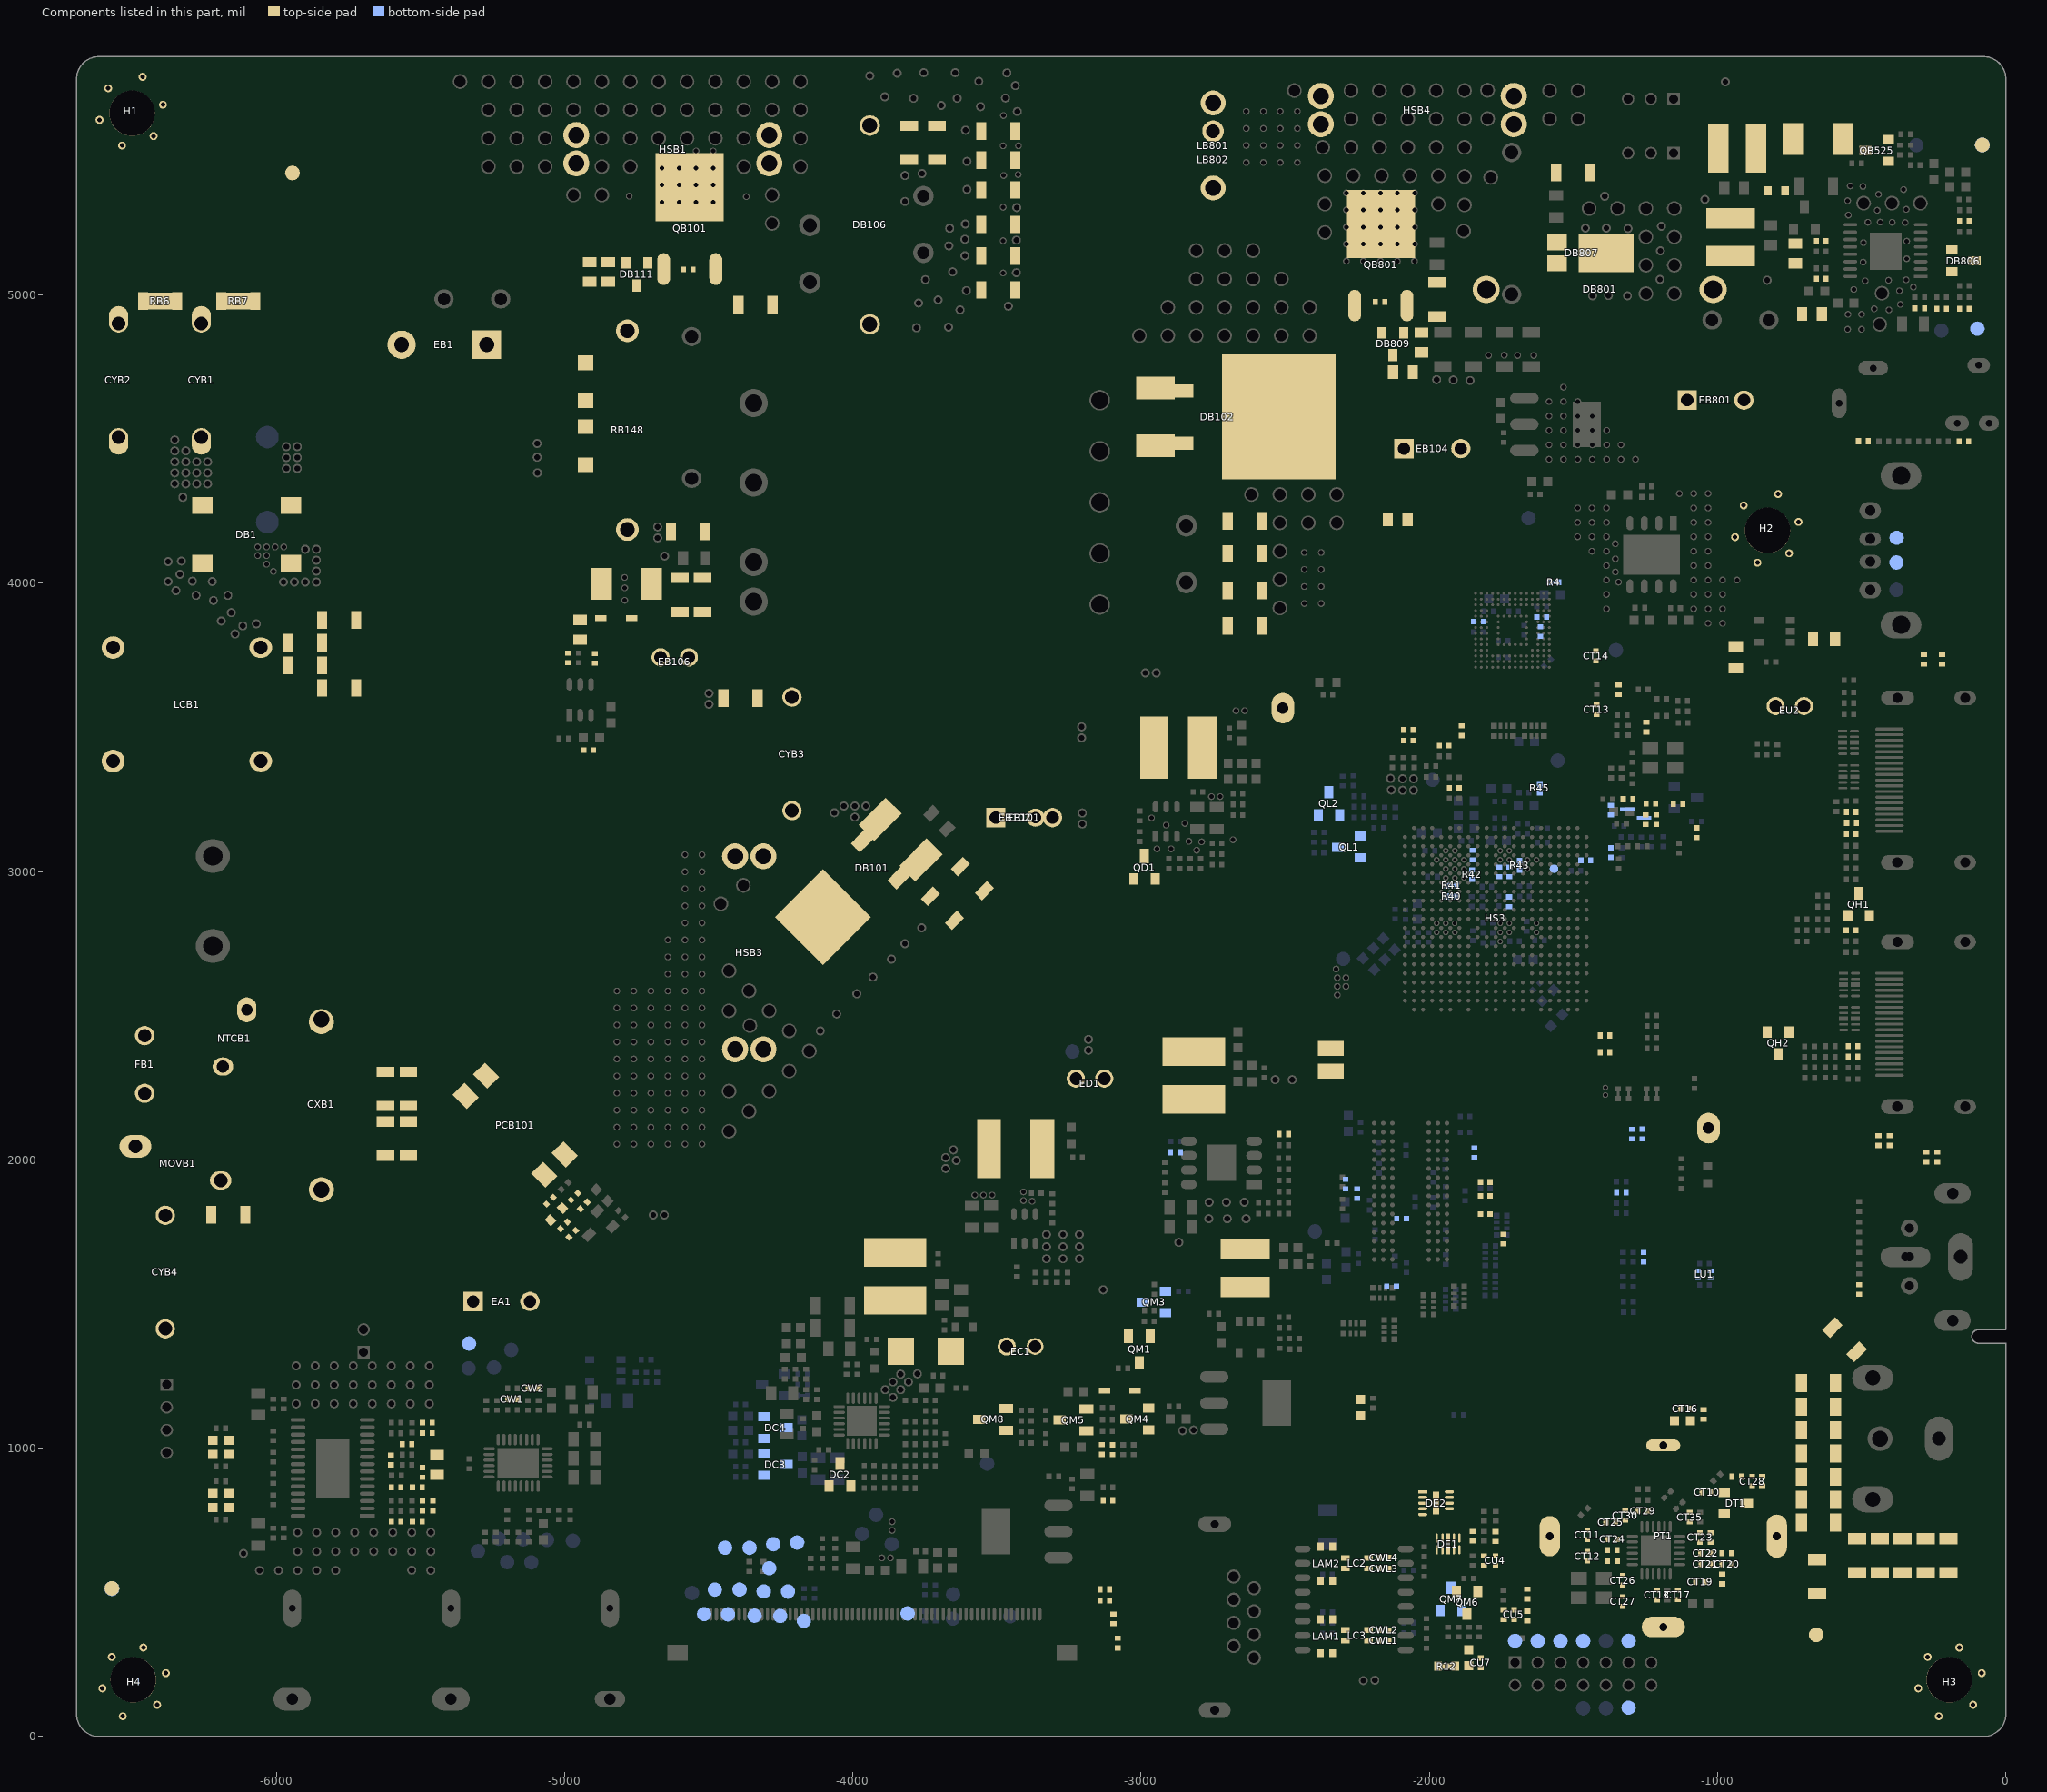
[diagram p0: the components of this part, seen from the top]
# Altium PCB MISC84395.PcbDoc (part 3 of 26)
Units mil, origin at the board's own origin, x right, y up, seen from the top; angles counter-clockwise.
Board outline 6692.91 x 5826.77 mil, 2 copper layers (TopLayer, BottomLayer), stack 61.855 mil thick; 951 components, 565 nets, 4374 pads, 1804 vias.
Unrouted connection lines stored in the file: 1.

## Components (designator, comment, footprint, x,y, rotation, side; value= is the part's Value field where it differs from the comment) (continued)
CT10 "0.1uF-0402-X5R-±20%-16V" C0402#1 -1037.15,847 r180 top
CT11 "30pF-0402-NPO-±5%-50V" C0402#1 -1452,699.54 r270 top
CT12 "30pF-0402-NPO-±5%-50V" C0402#1 -1452,625.26 r90 top
CT13 "0.022uF-0402-X7R-±10%-16V" C0402#1 -1419.65,3561.74 r90 top
CT14 "NC/0.1uF-0402-X5R-±20%-16V" C0402#1 -1422,3748 r90 top
CT15 "10uF-0603-X5R-±20%-6.3V" C0603 -1122,1095 r0 top
CT16 "0.1uF-0402-X5R-±20%-16V" C0402#1 -1112,1137 r0 top
CT17 "1uF-0402-X5R-±20%-6.3V" C0402#1 -1138.21,491.19 r90 top
CT18 "0.01uF-0402-X7R-±10%-50V" C0402#1 -1210.21,491.19 r270 top
CT19 "0.1uF-0402-X5R-±20%-16V" C0402#1 -1060,536 r0 top
CT20 "5.6pF-0402-NPO-±5%-50V" C0402#1 -968,597.69 r180 top
CT21 "1000pF-0402-X7R-±10%-50V" C0402#1 -1041,597.69 r180 top
CT22 "1000pF-0402-X7R-±10%-50V" C0402#1 -1041.43,635.73 r180 top
CT23 "0.1uF-0402-X5R-±20%-16V" C0402#1 -1061.25,690.46 r90 top
CT24 "0.1uF-0402-X5R-±20%-16V" C0402#1 -1365.07,683.98 r180 top
CT25 "1uF-0402-X5R-±20%-6.3V" C0402#1 -1371,743 r0 top
CT26 "NC/Ceramic capacitor,CAP MC,50V,5.6pF,±0.25pF,NPO,0402,SMD,TP" C0402#1 -1329.29,542 r270 top
CT27 "NC/Ceramic capacitor,CAP MC,50V,5.6pF,±0.25pF,NPO,0402,SMD,TP" C0402#1 -1329.29,468 r90 top
CT28 "1000pF-0402-X7R-±10%-50V" C0402#1 -880,885 r90 top
CT29 "0.1uF-0402-X5R-±20%-16V" C0402#1 -1259,783 r180 top
CT30 "1uF-0402-X5R-±20%-6.3V" C0402#1 -1321,767 r90 top
CT35 "0.1uF-0402-X5R-±20%-16V" C0402#1 -1097,761 r90 top
CT41 "4700pF-1206-X7R-±10%-1000V" C1206 -649.76,981.5 r0 top
CT42 "4700pF-1206-X7R-±10%-1000V" C1206 -649.76,821.5 r0 top
CT43 "4700pF-1206-X7R-±10%-1000V" C1206 -649.76,741.5 r0 top
CT44 "4700pF-1206-X7R-±10%-1000V" C1206 -649.76,1062.5 r0 top
CT45 "4700pF-1206-X7R-±10%-1000V" C1206 -655.34,554.41 r90 top
CT46 "4700pF-1206-X7R-±10%-1000V" C1206 -649.76,1143.5 r0 top
CT47 "NC/4700pF-1206-X7R-±10%-1000V" C1206 -516.38,626.94 r90 top
CT48 "NC/4700pF-1206-X7R-±10%-1000V" C1206 -649.76,1225.5 r0 top
CT49 "NC/4700pF-1206-X7R-±10%-1000V" C1206 -437.27,626.94 r90 top
CT50 "NC/10uF-0603-X5R-±20%-6.3V" C0603 -2238,1141 r90 top
CT55 "NC/4700pF-1206-X7R-±10%-1000V" C1206 -358.05,626.94 r90 top
CT60 "Ceramic capacitor,CAP MC,1KV,470pF,±5%,NPO,1206,SMD,TP" C1206 -649.76,901.5 r180 top
CT67 "NC/4700pF-1206-X7R-±10%-1000V" C1206 -278.94,626.94 r90 top
CT68 "NC/4700pF-1206-X7R-±10%-1000V" C1206 -199.65,626.94 r90 top
CT70 "NC/4700pF-1206-X7R-±10%-1000V" C1206 -560,1376.44 r315 top
CU "NC/10uF-0805-X5R-±20%-16V" C0805 -936.83,3742.97 r270 top
CU1 "10uF-0805-X5R-±20%-16V" C0805 -630.83,3806 r180 top
CU4 "0.01uF-0402-X7R-±10%-50V" C0402#1 -1771,610 r270 top
CU5 "0.01uF-0402-X7R-±10%-50V" C0402#1 -1706.34,422.89 r90 top
CU6 "10uF-0603-X5R-±20%-10V" C0603 -1864,273.81 r90 top
CU7 "NC/0.1uF-0402-X5R-±20%-16V" C0402#1 -1822,255.84 r90 top
"CVBS OUT" "TEST" TP#3 -1567.65,3009.74 r90 bottom
CW1 "Ceramic capacitor,CAP MC,50V,1000pF,±10%,X7R,0402,SMD,TP" C0402#1 -5181,1170 r180 top
CW2 "1uF-0402-X5R-±20%-6.3V" C0402#1 -5109.16,1208 r0 top
CWL1 "0.1uF-0402-X5R-±20%-16V" C0402#1 -2157,333 r180 top
CWL2 "0.1uF-0402-X5R-±20%-16V" C0402#1 -2157,369 r180 top
CWL3 "0.1uF-0402-X5R-±20%-16V" C0402#1 -2157,583 r180 top
CWL4 "0.1uF-0402-X5R-±20%-16V" C0402#1 -2157,620 r180 top
CXB1 "X capacitor,CAP X2,MP,280VAC,0.33uF,±10%,S,15mm,PC,DIP,JH" CAP18*8.5-V-15 -5843.63,2192 r90 top
CYB1 "Y capacitor,CAP Y1,CD,470pF,400VAC,±20%,KS,10mm,Y5U,DIP,Walsin" CAP13*5-V-10-1#1 -6260,4703.85 r90 top
CYB2 "Y capacitor,CAP Y1,CD,470pF,400VAC,±20%,KS,10mm,Y5U,DIP,Walsin" CAP13*5-V-10-1#1 -6547,4703.85 r90 top
CYB3 "Y capacitor,CAP Y1,CD,470pF,400VAC,±20%,KS,10mm,Y5U,DIP,Walsin" CAP13*5-V-10-1#2 -4211,3408.15 r270 top
CYB4 "NC/Y capacitor,CAP Y1,CD,470pF,400VAC,±20%,KS,10mm,Y5U,DIP,Walsin" CAP13*5-V-10-1#2 -6385,1611.15 r270 top
D4 "NC/SFI0402-240E-2R5PP-LF" DIODE-S0402 -1231.77,3235.74 r0 top
D5 "NC/TVS diode,DIO ESD,0.4pF,11V,SOD882,SMD,PESD5V0F1BL,NXP" DIODE-S0402 -1723.85,2895.54 r90 bottom
D11 "NC/TVS diode,DIO ESD,3pF,58V,0402,SMD,SDV1005H260C030YPTF,Sunlord" DIODE-S0402 -2881,2026 r180 bottom
D12 "NC/TVS diode,DIO ESD,3pF,58V,0402,SMD,SDV1005H260C030YPTF,Sunlord" DIODE-S0402 -2505,2090 r0 top
D13 "NC/TVS diode,DIO ESD,3pF,58V,0402,SMD,SDV1005H260C030YPTF,Sunlord" DIODE-S0402 -1343,3631 r270 top
D14 "NC/TVS diode,DIO ESD,3pF,58V,0402,SMD,SDV1005H260C030YPTF,Sunlord" DIODE-S0402 -1248,3500.73 r270 top
DA1 "NC/AIES12U020R2-D" DIODE-S0402 -1137,3235 r180 top
DA2 "NC/AIES12U020R2-D" DIODE-S0402 -1370,3213 r270 bottom
DB1 "Bridge rectifier,DIO BRD,3A,800V,YBS,SMD,YBS3010A,YJ" B/YBS3010A -6103,4169 r270 top
DB101 "Schottky diode,DIO SBD D1,10A,150V,TO-252,SMD,MBR10150GCT,PINGWEI" D2PAK3#1 -4040.54,2899.31 r45 top
DB102 "Schottky diode,DIO SBD D1,10A,150V,TO-263,SMD,HBR10150SS,JLHW" D2PAK3#2 -2654.83,4580.49 r180 top
DB104 "Rectifier diode,DIO SI S,1A,1000V,SMAF,SMD,M7F,YJ" DIODE-S-2 -4784.61,3998.3 r180 top
DB106 "Rectifier diode,DIO FRD S,1A,1000V,DO-41,DIP,FR107G,YJ" D1-H-17.5 -3941,5243 r90 top
DB109 "Rectifier diode,DIO FRD S,1.2A,800V,SOD-123FL,SMD,F1K,YJ" DIODE-S-14 -4927,4698.8 r90 top
DB110 "Rectifier diode,DIO FRD S,1.2A,800V,SOD-123FL,SMD,F1K,YJ" DIODE-S-14 -4927,4476.8 r90 top
DB111 "Switching diode,DIO SW D1,215mA,85V,SOT-23,SMD,KAV70,KEXIN" SO-23 -4748.97,5070.6 r0 top
DB121 "Switching diode,DIO SW S,200mA,250V,SOD-323,SMD,BAV21WS,BLUE ROCKET" DIODE-S-12 -4821,3879 r0 top
DB801 "NC/Schottky diode,DIO SBD S,3A,100V,DO-201AD,DIP,SR3100,YJ" D3-H-20 -1409.19,5019 r0 top
DB802 "NC/M7(WEJ)" DIODE-S-2 -653,5541 r180 top
DB806 "Switching diode,DIO SW D1,215mA,85V,SOT-23,SMD,KAV70,KEXIN" SO-23 -148,5118 r90 top
DB807 "NC/Schottky diode,DIO SBD S,3A,150V,TO-277,SMD,SBT03HL150T3TR,SL" DIODE-S-13 -1441.84,5145.22 r270 top
DB809 "NC/LBAV70LT1G(LRC)" SO-23 -2126.5,4829 r0 top
DBS7 "DOLBY PLUS" "DOLBY PLUS-SILK" -797,1546 r90 bottom
DC1 "Schottky diode,DIO SBD S,1A,40V,DO-214AC,SMD,SS14,PINGWEI" DIODE-S-1 -3747,1336 r0 top
DC2 "Switching diode,DIO SW D2,75V,SOT-23,SMD,KAV99,KEXIN" SO-23 -4045,909 r180 top
DC3 "Switching diode,DIO SW D2,75V,SOT-23,SMD,KAV99,KEXIN" SO-23 -4268,943.19 r270 bottom
DC4 "NC/BAV99-BR" SO-23 -4268,1071.19 r270 bottom
DE1 "NC/ULC0524P" RCL0524P -1935,668 r0 top
DE2 "NC/TVS diode,DIO ESD,3.6pF,18V,DFN2525P10E,SMD,AZ3133-04F,Amazing (OEM material)" DFN10/0.5-2 -1977,809.63 r0 top
DH1 "NC/ULCE0505A015FR" DIODE-S0402 -536.64,3206.79 r180 top
DH2 "NC/22pF-0402-NPO-±5%-50V" DIODE-S0402 -535.88,3168.79 r180 top
DH3 "NC/22pF-0402-NPO-±5%-50V" DIODE-S0402 -536.38,3130.29 r180 top
DH4 "NC/22pF-0402-NPO-±5%-50V" DIODE-S0402 -537.37,2796.16 r0 top
DH5 "NC/22pF-0402-NPO-±5%-50V" DIODE-S0402 -530.62,2394.24 r180 top
DH6 "NC/22pF-0402-NPO-±5%-50V" DIODE-S0402 -530.62,2357.24 r180 top
DI1 "NC/AVLC18S02003" DIODE-S0402 -3081,324 r270 top
DI2 "NC/AVLC18S02003" DIODE-S0402 -3096,408 r90 top
DI4 "NC/AVLC18S02003" DIODE-S0402 -3126,510 r180 top
DI04 "NC/AVLC18S02003" DIODE-S0402 -3126,472 r180 top
DK1 "NC/TVS diode,DIO ESD,3pF,58V,0402,SMD,SDV1005H260C030YPTF,Sunlord" DIODE-S0402 -1742.34,422.89 r90 top
DK3 "NC/AVLC18S02003" DIODE-S0402 -1811,610 r270 top
DM1 "Switching diode,DIO SW S,150mA,75V,SOD-323,SMD,1N4148WS,BLUE ROCKET" DIODE-S-12 -3074,1200 r0 top
DM2 "TEST" TP#2 -1309,332 r180 bottom
DM3 "TEST" TP#2 -380,4072 r90 bottom
DO1 "NC/NC/SFI0402-240E-2R5PP-LF" DIODE-S0402 -1333.8,1888 r0 bottom
DO7 "NC/SFI0402-240E-2R5PP-LF" DIODE-S0402 -509,1550.73 r270 top
DP2 "TEST" TP#2 -1309,100 r180 bottom
DP3 "TEST" TP#2 -379,4158 r90 bottom
DT1 "Switching diode,DIO SW D2,75V,SOT-23,SMD,KAV99,KEXIN" SO-23 -937,809 r90 top
DT2 "NC/AVLC18S02003" DIODE-S0402 -1365.16,608.98 r0 top
DT3 "NC/AVLC18S02003" DIODE-S0402 -1365.34,646.98 r0 top
DT4 "NC/?" DIODE-S0402 -846,885 r90 top
DU1 "NC/AIES12U020R2-D" DIODE-S0402 -1390.52,2372.74 r180 top
DU2 "NC/AIES12U020R2-D" DIODE-S0402 -1390.52,2431.74 r180 top
DU3 "NC/AIES12U020R2-D" DIODE-S0402 -284.39,3737 r270 top
DU4 "NC/AIES12U020R2-D" DIODE-S0402 -221.17,3737 r270 top
DU5 "NC/TVS diode,DIO ESD,8pF,10V,0402,SMD,AZ5725-01F.R7GR,Amazing" DIODE-S0402 -1660,494 r270 top
DU6 "NC/TVS diode,DIO ESD,8pF,10V,0402,SMD,AZ5725-01F.R7GR,Amazing" DIODE-S0402 -1660,418 r90 top
DU7 "NC/TVS diode,DIO ESD,8pF,10V,0402,SMD,AZ5725-01F.R7GR,Amazing" DIODE-S0402 -1771.01,694 r90 top
DU8 "NC/AIES12U020R2-D" DIODE-S0402 -403,2067 r270 top
DU9 "NC/AIES12U020R2-D" DIODE-S0402 -442,2067 r270 top
DV1 "NC/TVS diode,DIO ESD,8pF,10V,0402,SMD,AZ5725-01F.R7GR,Amazing" DIODE-S0402 -494.87,4492.69 r0 top
DV2 "NC/TVS diode,DIO ESD,8pF,10V,0402,SMD,AZ5725-01F.R7GR,Amazing" DIODE-S0402 -145.83,4492 r180 top
DV3 "NC/TVS diode,DIO ESD,8pF,10V,0402,SMD,AZ5725-01F.R7GR,Amazing" DIODE-S0402 -238,2010 r90 top
DV4 "NC/TVS diode,DIO ESD,8pF,10V,0402,SMD,AZ5725-01F.R7GR,Amazing" DIODE-S0402 -276,2010 r90 top
EA1 "Aluminium electrolytic capacitor,CAP AL,16V,470uF,±20%,PKRM,P,5.0mm,10×12.5,DIP,TP,Koshin" EC(10*12)-V-5 -5218.42,1509 r0 top locked
EB1 "Aluminium electrolytic capacitor,CAP AL,450V,82uF,±20%,SL,KL,BK,7.5mm,18×35.5,DIP,CapXon" EC(18*41)-H-7.5-1 -5417.37,4729 r0 top locked
EB101 "Aluminium electrolytic capacitor,CAP AL,25V,470uF,±20%,LD,PKLH,P,5.0mm,10×12.5,DIP,TP,Koshin" EC(10*12.5)-V-5#1 -3405.57,3187 r0 top
EB102 "NC/270uF-16V-±20%-8×11.5-105℃-PS-short pins-F=3.5(Capxon)" EC(8*11)-V-3.5 -3435.1,3187 r0 top
EB104 "Aluminium electrolytic capacitor,CAP AL,35V,330uF,±20%,LD,PKZF,P,5.0mm,10×12.5,DIP,TP,Koshin" EC(10*12.5)-V-5#2 -1989.47,4467 r0 top
EB106 "10uF-50V-±20%-5×11-105℃-GH-taped reel-F=2.5(CapXon)" EC(5*11)-V-2.5#1 -4617.79,3743 r0 top
EB801 "Aluminium electrolytic capacitor,CAP AL,63V,100uF,±20%,LD,PKLF,P,5.0mm,10×12.5,DIP,TP,Koshin" EC(10*12.5)-V-5#3 -1007.22,4635 r0 top locked
EC1 "Aluminium electrolytic capacitor,CAP AL,25V,100uF,±20%,LD,SY,P,2.5mm,6.3×7,DIP,TP,CapXon" EC(6.3*11)-V-2.5#1 -3417,1353 r0 top locked
ED1 "Aluminium electrolytic capacitor,CAP AL,10V,470uF,±20%,PKZH,P,2.5mm,6.3×11,DIP,TP,Koshin" EC(6.3*11)-V-2.5#2 -3177,2282 r0 top locked
EU2 "NC/Aluminium electrolytic capacitor,CAP AL,16V,100uF,±20%,RK,P,2.5mm,5×11,DIP,TP,XL" EC(5*11)-V-2.5#2 -749.83,3574 r0 top locked
EVA1 "NC/7×7×3mm-C-4305 fire-retardant foam-black" EVA(7*7*3) -4564,5234 r180 bottom
EVA2 "NC/7×7×3mm-C-4305 fire-retardant foam-black" EVA(7*7*3) -5784,2127 r180 bottom
EVA3 "NC/7×7×3mm-C-4305 fire-retardant foam-black" EVA(7*7*3) -2796,4546 r180 bottom
EVA4 "NC/7×7×3mm-C-4305 fire-retardant foam-black" EVA(7*7*3) -4161,2751 r90 bottom
EVA5 "NC/7×7×3mm-C-4305 fire-retardant foam-black" EVA(7*7*3) -4716,749 r180 bottom
EVA6 "NC/7×7×3mm-C-4305 fire-retardant foam-black" EVA(7*7*3) -1487.5,1231 r180 bottom
FB1 "Slow-blow fuse,FUSE T,P,3.15A,250VAC,8.4×4.0×7.2mm,DIP,TP,LS" "FUSE8.5*4-V-5(T3.15AL 250V~)" -6456.63,2331 r90 top
GD1 "NC/7.00×8.35mm-nylon-white-WQM" Fixed -6043.31,1515.75 r0 top locked
GD2 "NC/7.00×8.35mm-nylon-white-WQM" Fixed -5590.55,5492.13 r0 top locked
GD3 "NC/7.00×8.35mm-nylon-white-WQM" Fixed -4468.5,3307.09 r0 top locked
GD4 "NC/7.00×8.35mm-nylon-white-WQM" Fixed -3169.29,5492.13 r0 top locked
GL1 "Silicone,0.5g,general,60,white,SLD-8854W,XY" "Silica gel-15" -5827,3298 r0 top
GL2 "Silicone,0.5g,general,60,white,SLD-8854W,XY" "Silica gel-10" -6093,4703 r180 top
GND_JP1 "NC" GND -1313,3217.4 r180 bottom
GND_JP2 "NC" GND -1255,3186 r180 bottom
H1 "Location hole" ASSE4.0C-3 -6500,5629.92 r180 top locked
H2 "Location hole" ASSE4.0C-3 -826.77,4183.07 r180 top locked
H3 "Location hole" ASSE4.0C-3 -196.85,196.85 r0 top locked
H4 "Location hole" ASSE4.0C-3 -6496.06,196.85 r0 top locked
"High Voltage" "High Voltage" "High Voltage" -6075,2827 r0 top
HOT "HOT" HOT -5238.89,5625.83 r0 top
HS3 "Heat sink,40.0×40.0×2.3mm,AL6063,black,nano-carbon,wave-pattern type-bottom milled groove,pin length 6.0mm,Asink" HS(40*40*2.3)-1 -1770.17,2838.54 r270 top locked
HSB1 "NC/Heat sink,17.5×14.5×0.5mm,copper sheet,matte tin plated,natural,four pins,WT" HS149-YZ -4624.35,5505.21 r180 top
HSB3 "NC/Heat sink,17.5×14.5×0.5mm,copper sheet,matte tin plated,natural,four pins,WT" HS149-YZ -4359.21,2718.35 r270 top
HSB4 "NC/Heat sink,17.5×14.5×0.5mm,copper sheet,matte tin plated,natural,four pins,WT" HS149-YZ -2042,5641 r180 top
IR "TEST" TP#2 -1702.7,332 r180 bottom
KEY "TEST" TP#2 -1466.48,332 r180 bottom
L3 "GZ1005U121CTF(120ohm-500mA)" L0402 -1311.04,3250.74 r0 top
LAM1 "Common-mode choke,321620,60uH,H2.0mm,DCM321620F2SF-600T02,SMD,TAI-TECH" L/LC4/3.2*1.6 -2357,348 r270 top
LAM2 "Common-mode choke,321620,60uH,H2.0mm,DCM321620F2SF-600T02,SMD,TAI-TECH" L/LC4/3.2*1.6 -2357,600 r270 top
LB801 "Differential-mode inductor,Inductor,DR12×12,70uH,0.15×12P,38.5Ts,H13.5MAX,SYDR1212-L070uA,DIP,EDL" L/LC2/15*14.5-V7.5 -2750.11,5518.36 r90 top
LB802 "NC/Differential-mode inductor,Inductor,DR12×14,68uH,0.45,20Ts,H13.5MAX,SYDR1214-L068uA,DIP,Soldier" L(13.5*15.5)-V-5 -2750.11,5469.15 r90 top
LB804 "Power inductor,2.2uH,±20%,2A,0.28×1P,DR4.5×3.2,SMD,PIO43-2R2MTP02,FH" L(4.5*3.5)-S -955,5200 r90 top
LB805 "Power inductor,2.2uH,±20%,2A,0.28×1P,DR4.5×3.2,SMD,PIO43-2R2MTP02,FH" L(4.5*3.5)-S -932,5508 r0 top
LBA1 "Ferrite bead,BEAD,600ohm,0603,2A,SMD,TP,EPZ1608E601-2R0TF,Sunlord" L0603 -6192.02,794.06 r180 top
LBA2 "Ferrite bead,BEAD,600ohm,0603,2A,SMD,TP,EPZ1608E601-2R0TF,Sunlord" L0603 -6192.02,843.06 r180 top
LBA3 "Ferrite bead,BEAD,600ohm,0603,2A,SMD,TP,EPZ1608E601-2R0TF,Sunlord" L0603 -6192.02,979.06 r180 top
LBA4 "Ferrite bead,BEAD,600ohm,0603,2A,SMD,TP,EPZ1608E601-2R0TF,Sunlord" L0603 -6192.08,1027 r180 top
LC "TEST" TP#2 -5331,1363 r180 bottom
LC1 "Power inductor,22uH,±10%,1.7A,0.27×1P,DR5.8×4.5,SMD,CKO54-22uH/M-B30,CK" L(5.8*4.5)-S -3853,1596 r90 top
LC2 "Common-mode choke,2012,800ohm,H1.2mm,WCM2012F2SF-801-N,SMD,TAI-TECH" L/LC4/2*1.2-S -2251,601 r180 top
LC3 "Common-mode choke,2012,800ohm,H1.2mm,WCM2012F2SF-801-N,SMD,TAI-TECH" L/LC4/2*1.2-S -2251,351 r180 top
LCB1 "Common-mode choke,UU10.5,18mH MIN,0.35×1P,80Ts,H14.5MAX,SYUU10.5-L002,DIP,CK" L/UU10.5/10*13-2 -6309.91,3579.85 r90 top
LD1 "Power inductor,4.7uH,±20%,2.8A,0.32×1P,DR5.8×4.5,SMD,CKO54-4.7uH/M,CK" L(6.0*4.5)-S -3435,2039 r0 top
LD2 "Power inductor,2.2uH,±20%,3A,0.4×1P,DR5.8×4.5,SMD,DSB5845-2R2M-LF,BLDX" L(5.8*4.5)-S -2817,2293 r270 top
LD3 "Power inductor,2.2uH,±20%,3A,0.4×1P,DR5.8×4.5,SMD,DSB5845-2R2M-LF,BLDX" L(5.8*4.5)-S -2871,3430.19 r180 top
LD5 "Power inductor,2.2uH,±20%,2A,0.28×1P,DR4.5×3.2,SMD,PIO43-2R2MTP02,FH" L(4.5*3.5)-S -2639,1624.26 r90 top
LED_R "TEST" TP#2 -1545.28,331.94 r90 bottom
LED_R_OFF "TEST" TP#2 -1624.02,331.94 r90 bottom
LG02 "0ohm-0402-±5%-1/16W" L0402 -3115,819 r0 top
LT1 "GZ1005U102CTF(1000ohm-300mA)" L0402 -1024.29,690 r270 top
LT2 "SDCL1005CR33JTDF" L0402 -933.73,901 r180 top
LT5 "SDCL1005C33NJTDF(Sunlord)" L0402 -984,546 r90 top
LT6 "SDCL1005C33NJTDF(Sunlord)" L0402 -967.91,635.76 r0 top
LT20 "Ferrite bead,BEAD,120ohm,0402,800mA,SMD,TP,CBM100505U121T,FH" L0402 -1049,1117 r270 top
LU1 "NC/DLP11SN900HL2" L/LC4/1.25*1.0 -1046,1603 r270 bottom
M1 "MARK" MARK -658,353 r0 top
M2 "MARK" MARK -82,5520 r0 top
M3 "MARK" MARK -5944,5423 r0 top
M4 "MARK" MARK -6570,514 r0 top
M5 "MARK" MARK -6570,513 r180 bottom
M6 "MARK" MARK -82,5520 r180 bottom
MAC "MAC" Barcode -4044,1787 r0 bottom
Manufacture_Info "Manufacture_Info" Manufacture_Info -3788,2286 r0 top
ML1 "NC/Latest Mylar sheet" Mylar -5411,3265 r90 top
MLV0N "TEST" TP#1 -4225,503 r0 bottom
MLV0P "TEST" TP#1 -4170,401.34 r0 bottom
MLV1N "TEST" TP#1 -4276,667 r270 bottom
MLV1P "TEST" TP#1 -4193,673 r270 bottom
MLV2N "TEST" TP#1 -4252,418 r270 bottom
MLV2P "TEST" TP#1 -4290,584 r270 bottom
MLV3N "TEST" TP#1 -4443,655 r90 bottom
MLV3P "TEST" TP#1 -4358.28,654.48 r90 bottom
MLV4N "TEST" TP#1 -4478.28,509.48 r90 bottom
MLV4P "TEST" TP#1 -4393,510 r90 bottom
MLV5N "TEST" TP#1 -4515.72,424.49 r180 bottom
MLV5P "TEST" TP#1 -4433,424 r180 bottom
MLVCKN "TEST" TP#1 -4341,419 r0 bottom
MLVCKP "TEST" TP#1 -4309.04,503.47 r0 bottom
MOVB1 "Varistor,VARISTOR,128J,680V,4000A,S,7.5mm,10mm,DIP,Thinking" VR(13*5)-V-7.5 -6340.64,1988.06 r180 top
MR300 "56ohm-0402-±1%-1/16W" R0402 -1806.07,1875.45 r0 top
MR301 "56ohm-0402-±1%-1/16W" R0402 -1806.07,1923.58 r0 top
MR313 "240ohm-0402-±1%-1/16W" R0402 -1806.07,1812.46 r180 top
NTCB1 "SCK102R55AMBY502(short pins/Weiqin)" NTC(10*5)-V5 -6143.63,2422 r90 top
P1 "NC/Conductive silicone,3×2×2.5mm,Black,Silicone Rubber,SMD,Joinset" "Silica gel(3*2*2.5)" -2342,2347 r90 top
PCB101 "LTV-817S-TA-B(Lite-On)" OC4-S-1 -5170.94,2120.23 r45 top
POL "TEST" TP#1 -3810,427 r90 bottom
PT1 "NC/Shield can,tinplate,natural,20.3×16.3×6mm,with sealing,LHD" SHIELD(16*20*6) -795,695 r90 top locked
PWM_DIM "NC/TEST" TP_BL -99,4883 r270 bottom
QB101 "MOSFET,NMOS,5A,700V,0.8Ω@ID=2.5A@VGS=10V,TO-252-2L,SVS5N70D,SL" TO-252-GDS -4565.71,5373 r0 top
QB525 "General transistor,Dynatron,NPN,0.2A,40V,60-300,SOT-23,KMBT3904,KEXIN" SOT-23 -449,5501 r270 top
QB801 "MOSFET,NMOS,15A,100V,0.105ohm@ID=6A@VGS=10V,TO-252,PA110BDA,UNIKC" TO-252-GDS -2168.29,5246.46 r0 top
QD1 "MOSFET,NMOS,0.3A,60V,3.3ohm@ID=0.5A@VGS=10V,SOT-23,2N7002K1,BLUE ROCKET" SOT-23-7 -2988,3014.19 r0 top
QH1 "General transistor,Dynatron,NPN,0.2A,40V,30-300,SOT-23,MMBT3904(f≥350MHz),BLUE ROCKET" SOT-23 -510.83,2887 r180 top
QH2 "General transistor,Dynatron,NPN,0.2A,40V,30-300,SOT-23,MMBT3904(f≥350MHz),BLUE ROCKET" SOT-23 -790,2404.03 r0 top
QL1 "General transistor,Dynatron,NPN,0.2A,40V,30-300,SOT-23,MMBT3904(f≥350MHz),BLUE ROCKET" SOT-23 -2279,3085 r90 bottom
QL2 "NC/General transistor,Dynatron,NPN,0.2A,40V,30-300,SOT-23,MMBT3904(f≥350MHz),BLUE ROCKET" SOT-23 -2348,3237 r0 bottom
QM1 "MOSFET,PMOS,-4.2A,-30V,0.052ohm@ID=-4.2A@VGS=-10V,SOT-23-3,AO3401,BLUE ROCKET" SOT-23-1 -3006,1342 r0 top
QM3 "General transistor,Dynatron,NPN,0.2A,40V,30-300,SOT-23,MMBT3904(f≥350MHz),BLUE ROCKET" SOT-23 -2955.97,1507.5 r90 bottom
QM4 "General transistor,Dynatron,NPN,0.2A,40V,30-300,SOT-23,MMBT3904(f≥350MHz),BLUE ROCKET" SOT-23 -3013,1101 r270 top
QM5 "MOSFET,PMOS,-4.3A,-30V,0.048ohm@ID=-3A@VGS=-4.5V,SOT-23-3L,NCE3407AY,NCEPOWER" SOT-23-1 -3237,1098 r270 top
QM6 "General transistor,Dynatron,NPN,0.2A,40V,30-300,SOT-23,MMBT3904(f≥350MHz),BLUE ROCKET" SOT-23 -1869,464 r0 top
QM7 "General transistor,Dynatron,NPN,0.2A,40V,30-300,SOT-23,MMBT3904(f≥350MHz),BLUE ROCKET" SOT-23 -1925,478 r0 bottom
QM8 "MOSFET,PMOS,-4.2A,-30V,0.052ohm@ID=-4.2A@VGS=-10V,SOT-23-3,AO3401,BLUE ROCKET" SOT-23-1 -3516,1100 r270 top
R1 "Thick film resistor,RES,1/16W,100ohm,±5%,0402,SMD" R0402 -1262,2090 r90 bottom
R2 "Thick film resistor,RES,1/16W,100ohm,±5%,0402,SMD" R0402 -1297.65,2089.87 r90 bottom
R3 "0ohm-0402-±5%-1/16W" R0402 -1249.77,3179.74 r270 top
R4 "NC/0ohm-0402-PCB" R0402SC#1 -1567.73,4003 r180 bottom
R5 "22ohm-0402-±5%-1/16W" R0402 -1887.71,3488.34 r270 top
R9 "10Kohm-0402-±5%-1/16W" R0402 -1610.65,3882.74 r0 bottom
R10 "NC/10Kohm-0402-±5%-1/16W" R0402 -1614.85,3832.74 r270 bottom
R11 "NC/10Kohm-0402-±5%-1/16W" R0402 -1829.65,3866.74 r0 bottom
R12 "NC/0ohm-0603-PCB" R0603SC -1940,244 r0 top
R21 "NC/1Kohm-0402-±5%-1/16W" R0402 -1212.77,3179.74 r90 top
R26 "68ohm-0402-±5%-1/16W" R0402 -1457.65,3038.74 r180 bottom
R27 "11Kohm-0402-±1%-1/16W" R0402 -3099,995 r90 top
R28 "1Kohm-0402-±5%-1/16W" R0402 -3136,995.27 r270 top
R30 "4K7ohm-0402-±5%-1/16W" R0402 -1257,1662.11 r90 bottom
R33 "4K7ohm-0402-±5%-1/16W" R0402 -1370.65,3065.74 r270 bottom
R34 "4K7ohm-0402-±5%-1/16W" R0402 -1073,3135 r270 top
R37 "4K7ohm-0402-±5%-1/16W" R0402 -1850,695 r90 top
R38 "0ohm-0402-±5%-1/16W" R0402 -1757.48,2998.72 r270 bottom
R39 "0ohm-0402-±5%-1/16W" R0402 -1722.48,2998.72 r270 bottom
R40 "NC/0ohm-0402-PCB" R0402SC#1 -1922.71,2914.51 r0 bottom
R41 "NC/0ohm-0402-PCB" R0402SC#1 -1922.48,2951.72 r0 bottom
R42 "NC/0ohm-0402-PCB" R0402SC#1 -1851.48,2989.72 r270 bottom
R43 "NC/0ohm-0402-PCB" R0402SC#1 -1686.97,3021.58 r270 bottom
R45 "NC/0ohm-0402-PCB" R0402SC#2 -1617.27,3288.74 r270 bottom
R46 "1Kohm-0402-±1%-1/16W" R0402 -2073,3454 r180 top
R47 "1Kohm-0402-±1%-1/16W" R0402 -1913.28,3290.48 r180 top
R48 "1Kohm-0402-±1%-1/16W" R0402 -2073,3491 r0 top
R49 "1Kohm-0402-±1%-1/16W" R0402 -1948.65,3436.74 r0 top
R50 "240ohm-0402-±1%-1/16W" R0402 -1850,3057.27 r90 bottom
R51 "1Kohm-0402-±1%-1/16W" R0402 -2250.28,1882.97 r270 bottom
R52 "1Kohm-0402-±1%-1/16W" R0402 -2290.97,1916.32 r270 bottom
R53 "33ohm-0402-±5%-1/16W" R0402 -2096.07,1796.71 r0 bottom
R54 "0ohm-0402-±5%-1/16W" R0402 -2130.87,1561.48 r0 bottom
R55 "0ohm-0402-±5%-1/16W" R0402 -1742.9,1725.53 r90 top
R56 "0ohm-0402-±5%-1/16W" R0402 -1843.79,2024.88 r90 bottom
RA5 "NC/1Kohm-0402-±5%-1/16W" R0402 -5492.6,799.99 r270 top
RA6 "1Kohm-0402-±5%-1/16W" R0402 -5456.6,799.94 r270 top
RA8 "NC/100Kohm-0402-±5%-1/16W" R0402 -5583.86,863.93 r0 top
RA11 "12Kohm-0402-±1%-1/16W" R0402 -5602.61,959.21 r90 top
RA12 "NC/1Kohm-0402-±5%-1/16W" R0402 -5475.94,1053 r180 top
RA13 "1Kohm-0402-±5%-1/16W" R0402 -5475.94,1089 r180 top
RA19 "NC/47Kohm-0402-±5%-1/16W" R0402 -5510.6,863.94 r180 top
RA21 "NC/20Kohm-0402-±1%-1/16W" R0402 -5546.6,1013.94 r180 top
RA25 "NC/10ohm-0402-±5%-1/16W" R0402 -5492.6,915.94 r270 top
RA27 "10ohm-0805-±5%-1/8W" R0805 -5442.6,941.94 r270 top
RA31 "4K7ohm-0402-±5%-1/16W" R0402 -5510.6,744.94 r180 top
RA32 "4K7ohm-0402-±5%-1/16W" R0402 -5583.86,744.94 r0 top
RB1 "1M2ohm-1206-±5%-1/4W" R1206 -5541.63,2074.06 r90 top
RB2 "1M2ohm-1206-±5%-1/4W" R1206 -5621.63,2074.06 r90 top
RB3 "1M2ohm-1206-±5%-1/4W" R1206 -5541.63,2246.06 r90 top
RB4 "1M2ohm-1206-±5%-1/4W" R1206 -5621.63,2246.06 r90 top
RB5 "20ohm-1206-±5%-1/4W" R1206 -6166.25,1809.96 r0 top
RB6 "NC/0ohm-1206-PCB-D" R1206SC -6403,4978.68 r0 top
RB7 "NC/0ohm-1206-PCB-D" R1206SC -6132,4978.68 r0 top
RB101 "330Kohm-1206-±5%-1/4W" R1206 -5899.89,3715 r0 top
RB102 "330Kohm-1206-±5%-1/4W" R1206 -5781.94,3637 r180 top
RB103 "Thick film resistor,RES,1/8W,6.8Kohm,±1%,0805,SMD" R0402 -4988.43,3740.82 r270 top
RB104 "47Kohm-0402-±1%-1/16W" R0402 -4915.76,3421.3 r180 top
RB105 "510ohm-0402-±1%-1/16W" R0402 -4894.49,3739.57 r90 top
RB106 "68ohm-0805-±5%-1/8W" R0805 -4847.47,5079.78 r90 top
RB107 "20ohm-0805-±5%-1/8W" R0805 -4912.57,5079.78 r90 top
RB109 "10Kohm-0402-±1%-1/16W" R0402 -4571.27,5088 r180 top
RB114 "4R7ohm-1206-±1%-1/4W" R1206 -4600,3959.35 r270 top
RB115 "NC/4R7ohm-1206-±5%-1/4W" R1206 -4521.16,3959.17 r270 top
RB116 "NC/10ohm-1206-±5%-1/4W" R1206 -4572.06,4179.3 r0 top
RB117 "10ohm-1206-±5%-1/4W" R1206 -3708,5527 r90 top
RB118 "10ohm-1206-±5%-1/4W" R1206 -3804.34,5527.43 r90 top
RB119 "10ohm-1206-±5%-1/4W" R1206 -4337.94,4966 r0 top
RB121 "Thick film resistor,RES,1/8W,27Kohm,±1%,0805,SMD" R0805 -4946.49,3838.3 r270 top
RB124 "68ohm-1206-±5%-1/4W" R1206 -2640.89,3975 r0 top
RB125 "68ohm-1206-±5%-1/4W" R1206 -2640.89,3852 r0 top
RB126 "68ohm-1206-±5%-1/4W" R1206 -2640.89,4216 r0 top
RB128 "47ohm-1206-±5%-1/4W" R1206 -3585.25,2975.8 r315 top
RB129 "47ohm-1206-±5%-1/4W" R1206 -3689.24,2872.24 r315 top
RB130 "20ohm-1206-±5%-1/4W" R1206 -4390,3601 r0 top
RB131 "Thick film resistor,RES,1/10W,2Kohm,±1%,0603,SMD" R0603 -5028,1812 r225 top
RB132 "Thick film resistor,RES,1/16W,1.2Kohm,±1%,0402,SMD" R0402 -4965.17,1872.83 r225 top
RB133 "10Kohm-0402-±1%-1/16W" R0402 -4933.17,1841.83 r225 top
RB134 "4K7ohm-0402-±1%-1/16W" R0402 -4973,1744 r45 top
RB135 "18Kohm-0402-±1%-1/16W" R0402 -5002,1773 r45 top
RB136 "68ohm-1206-±5%-1/4W" R1206 -2640.89,4102 r0 top
RB140 "51Kohm-0805-±1%-1/8W" R0805 -2109.91,4221 r0 top
RB141 "2Mohm-1206-±5%-1/4W" R1206 -5900.27,3794 r180 top
RB142 "2Mohm-1206-±5%-1/4W" R1206 -5781.94,3873 r180 top
RB148 "Metal oxide film resistor,RES MOF,2WS,0.36ohm,±5%,DIP,TP,Royalohm" R2-H-17.5 -4782,4530.74 r90 top
RB151 "150Kohm-1206-±5%-1/4W" R1206 -3495.61,5364 r0 top
RB152 "150Kohm-1206-±5%-1/4W" R1206 -3495.61,5134.76 r180 top
RB153 "150Kohm-1206-±5%-1/4W" R1206 -3495.61,5017.37 r180 top
RB154 "150Kohm-1206-±5%-1/4W" R1206 -3495.61,5467.37 r0 top
RB155 "150Kohm-1206-±5%-1/4W" R1206 -3495.61,5568.37 r0 top
RB156 "150Kohm-1206-±5%-1/4W" R1206 -3495.61,5244.37 r180 top
RB158 "NC/Thick film resistor,RES,1/16W,51ohm,±1%,0402,SMD" R0402 -5050.95,1858.16 r225 top
RB801 "1Kohm-0402-±5%-1/16W" R0402 -144.27,4952.32 r180 top
RB802 "10Kohm-0402-±5%-1/16W" R0402 -223,4952.32 r180 top
RB803 "Thick film resistor,RES,1/16W,8.66Kohm,±1%,0402,SMD" R0402 -640.51,5186.52 r0 top
RB804 "270ohm-0402-±5%-1/16W" R0402 -299.46,4953.32 r0 top
RB805 "1Kohm-0402-±5%-1/16W" R0402 -640.73,5056 r0 top
RB806 "NC/30Kohm-0603-±5%-1/10W" R0603 -796,5361 r0 top
RB807 "20ohm-0805-±5%-1/8W" R0805 -2028,4835 r90 top
RB808 "10Kohm-0402-±5%-1/16W" R0402 -2170.47,4976 r0 top
RB809 "NC/10ohm-0805-±5%-1/8W" R0805 -2091.91,4732 r180 top
RB810 "10ohm-1206-±5%-1/4W" R1206 -1973,4984.06 r270 top
RB811 "10ohm-1206-±5%-1/4W" R1206 -1500.94,5424 r0 top
RB812 "NC/15Kohm-0402-±1%-1/16W" R0402 -144.69,5256.13 r0 top
RB814 "Thick film resistor,RES,1/8W,330Kohm,±1%,0805,SMD" R0805 -730,5144 r270 top
RB816 "2R2ohm-0805-±5%-1/8W" R0805 -672.5,4934 r180 top